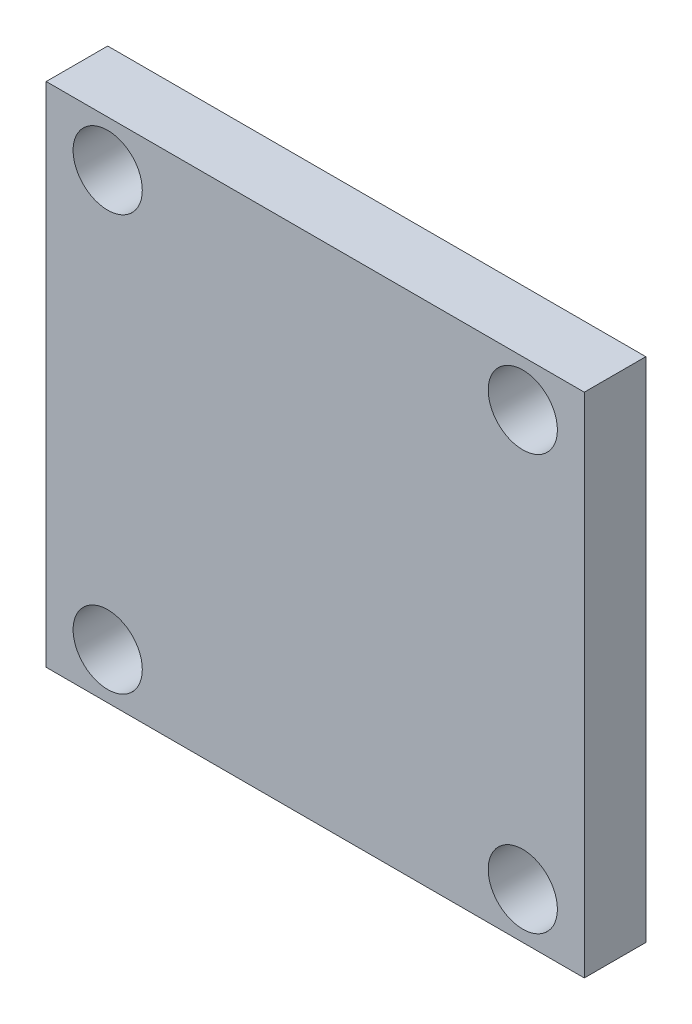
from build123d import *

# Parameters (mm, degrees)
SKETCH1_W                = 35
SKETCH1_H                = 33
BOSS_EXTRUDE1_DEPTH      = 4
M4_CLEARANCE_HOLE1_D     = 4.5
M4_CLEARANCE_HOLE1_DEPTH = 15
M4_CLEARANCE_HOLE1_TIP   = 1.351936393


with BuildPart() as part:
    # Sketch1 → Boss-Extrude1 (new body)
    with BuildSketch(Plane.XY):
        Rectangle(SKETCH1_W, SKETCH1_H)
    extrude(amount=BOSS_EXTRUDE1_DEPTH)

    # M4 Clearance Hole1
    with Locations(Plane.XY.offset(4)):
        with Locations((13.5, 13.5), (-13.5, 13.5), (-13.5, -13.5), (13.5, -13.5)):
            Hole(M4_CLEARANCE_HOLE1_D / 2, depth=M4_CLEARANCE_HOLE1_DEPTH)
            with Locations((0, 0, -(M4_CLEARANCE_HOLE1_DEPTH + M4_CLEARANCE_HOLE1_TIP / 2))):  # 118° drill point
                Cone(0, M4_CLEARANCE_HOLE1_D / 2, M4_CLEARANCE_HOLE1_TIP, mode=Mode.SUBTRACT)


solid = part.part
